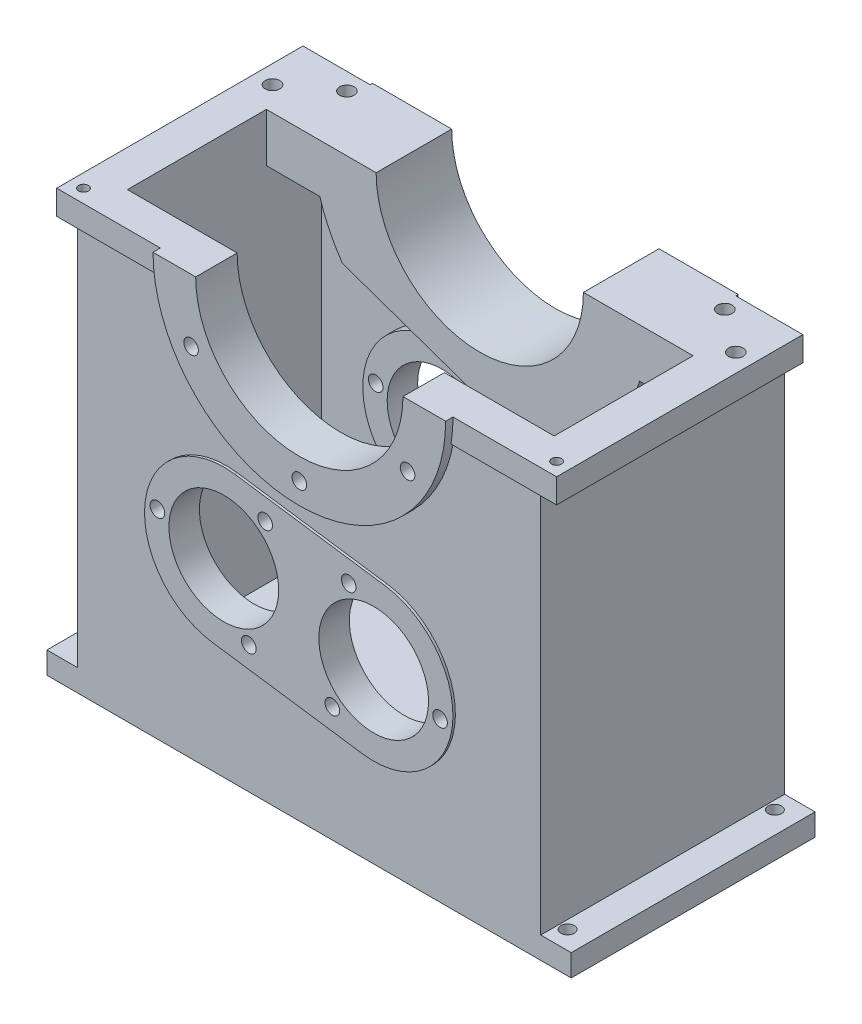
from build123d import *

# Parameters (mm, degrees)
BOSS_EXTRUDE1_DEPTH            = 2
BOSS_EXTRUDE2_DEPTH            = 100
SKETCH3_W                      = 380
SKETCH3_H                      = 200
BOSS_EXTRUDE3_DEPTH            = 232
SKETCH4_W                      = 395
SKETCH4_H                      = 202
BOSS_EXTRUDE4_DEPTH            = 20
SKETCH5_W                      = 202
SKETCH5_H                      = 20
BOSS_EXTRUDE5_DEPTH            = 15
BOSS_EXTRUDE6_START            = 6
BOSS_EXTRUDE6_DEPTH            = 6
SKETCH7_W                      = 200
SKETCH7_H                      = 18
BOSS_EXTRUDE7_DEPTH            = 25
SKETCH8_W                      = 200
SKETCH8_H                      = 18
BOSS_EXTRUDE8_DEPTH            = 25
SKETCH9_W                      = 350
SKETCH9_H                      = 114
CUT_EXTRUDE1_DEPTH             = 337
SKETCH10_W                     = 350
SKETCH10_H                     = 297
CUT_EXTRUDE2_DEPTH             = 45
SKETCH11_W                     = 350
SKETCH11_H                     = 297
CUT_EXTRUDE3_DEPTH             = 11
BOSS_EXTRUDE9_DEPTH            = 2
BOSS_EXTRUDE10_DEPTH           = 45
BOSS_EXTRUDE11_DEPTH           = 11
BOSS_EXTRUDE12_START           = 2
BOSS_EXTRUDE12_DEPTH           = 2
BOSS_EXTRUDE13_START           = 8
BOSS_EXTRUDE13_DEPTH           = 8
BOSS_EXTRUDE14_DEPTH           = 8
F_16_0_16_DIAMETER_HOLE1_D     = 16
F_16_0_16_DIAMETER_HOLE1_DEPTH = 30
F_12_0_12_DIAMETER_HOLE1_D     = 12
F_12_0_12_DIAMETER_HOLE1_DEPTH = 34
HOLE1_D                        = 170
HOLE1_DEPTH                    = 34
HOLE2_D                        = 170
F_11_0_11_DIAMETER_HOLE1_D     = 11
F_11_0_11_DIAMETER_HOLE1_DEPTH = 18
F_12_0_12_DIAMETER_HOLE2_D     = 12
F_12_0_12_DIAMETER_HOLE2_DEPTH = 12
F_8_0_8_DIAMETER_HOLE1_D       = 8
F_8_0_8_DIAMETER_HOLE1_DEPTH   = 12
F_12_0_12_DIAMETER_HOLE3_D     = 12
F_12_0_12_DIAMETER_HOLE3_DEPTH = 15
F_12_0_12_DIAMETER_HOLE4_D     = 12
F_12_0_12_DIAMETER_HOLE4_DEPTH = 25
F_12_0_12_DIAMETER_HOLE5_D     = 12
F_12_0_12_DIAMETER_HOLE5_DEPTH = 31
M80_CLEARANCE_HOLE1_D          = 90
M80_CLEARANCE_HOLE1_DEPTH      = 25
M80_CLEARANCE_HOLE2_D          = 90
FILLET1_R                      = 100


with BuildPart() as part:
    # Sketch1 → Boss-Extrude1 (new body)
    with BuildSketch(Plane.XY.offset(-156.692981355)):
        with BuildLine():
            Line((639.552238246, 214.743963655), (402.909046922, 214.743963655))
            ThreePointArc((402.909046922, 214.743963655), (521.230642584, 114.743963655), (639.552238246, 214.743963655))
        make_face()
    extrude(amount=-BOSS_EXTRUDE1_DEPTH)

    # Sketch2 → Boss-Extrude2 (add)
    with BuildSketch(Plane(origin=(0, 214.743963655, 0), x_dir=(1, 0, 0), z_dir=(0, 1, 0))):
        Polygon((331.230642584, 158.692981355), (521.230642584, 158.692981355), (711.230642584, 158.692981355), (711.230642584, 358.692981355), (331.230642584, 358.692981355), align=None)
    extrude(amount=-BOSS_EXTRUDE2_DEPTH)

    # Sketch3 → Boss-Extrude3 (add)
    with BuildSketch(Plane.XZ.offset(-114.743963655)):
        with Locations((521.230642584, -258.692981355)):
            Rectangle(SKETCH3_W, SKETCH3_H)
    extrude(amount=BOSS_EXTRUDE3_DEPTH)

    # Sketch4 → Boss-Extrude4 (add)
    with BuildSketch(Plane(origin=(0, 214.743963655, 0), x_dir=(-1, 0, 0), z_dir=(0, 1, 0))):
        with Locations((-513.730642584, -257.692981355)):
            Rectangle(SKETCH4_W, SKETCH4_H)
    extrude(amount=BOSS_EXTRUDE4_DEPTH)

    # Sketch5 → Boss-Extrude5 (add)
    with BuildSketch(Plane(origin=(711.230642584, 0, 0), x_dir=(0, 0, -1), z_dir=(1, 0, 0))):
        with Locations((257.692981355, 224.743963655)):
            Rectangle(SKETCH5_W, SKETCH5_H)
    extrude(amount=BOSS_EXTRUDE5_DEPTH)

    # Sketch6 → Boss-Extrude6 (add)
    with BuildSketch(Plane.XY.offset(-156.692981355).offset(BOSS_EXTRUDE6_START)):
        with BuildLine():
            Line((401.230642584, 234.743963655), (641.230642584, 234.743963655))
            ThreePointArc((641.230642584, 234.743963655), (521.230642584, 114.743963655), (401.230642584, 234.743963655))
        make_face()
    extrude(amount=-BOSS_EXTRUDE6_DEPTH)

    # Sketch7 → Boss-Extrude7 (add)
    with BuildSketch(Plane.ZY.offset(-331.230642584)):
        with Locations((-258.692981355, -108.256036345)):
            Rectangle(SKETCH7_W, SKETCH7_H)
    extrude(amount=BOSS_EXTRUDE7_DEPTH)

    # Sketch8 → Boss-Extrude8 (add)
    with BuildSketch(Plane(origin=(711.230642584, 0, 0), x_dir=(0, 0, -1), z_dir=(1, 0, 0))):
        with Locations((258.692981355, -108.256036345)):
            Rectangle(SKETCH8_W, SKETCH8_H)
    extrude(amount=BOSS_EXTRUDE8_DEPTH)

    # Sketch9 → Cut-Extrude1 (cut)
    with BuildSketch(Plane(origin=(0, 234.743963655, 0), x_dir=(-1, 0, 0), z_dir=(0, 1, 0))):
        with Locations((-521.230642584, -241.692981355)):
            Rectangle(SKETCH9_W, SKETCH9_H)
    extrude(amount=-CUT_EXTRUDE1_DEPTH, mode=Mode.SUBTRACT)

    # Sketch10 → Cut-Extrude2 (cut)
    with BuildSketch(Plane.XY.offset(-298.692981355)):
        with Locations((521.230642584, 46.243963655)):
            Rectangle(SKETCH10_W, SKETCH10_H)
    extrude(amount=-CUT_EXTRUDE2_DEPTH, mode=Mode.SUBTRACT)

    # Sketch11 → Cut-Extrude3 (cut)
    with BuildSketch(Plane(origin=(0, 0, -184.692981355), x_dir=(-1, 0, 0), z_dir=(0, 0, -1))):
        with Locations((-521.230642584, 46.243963655)):
            Rectangle(SKETCH11_W, SKETCH11_H)
    extrude(amount=-CUT_EXTRUDE3_DEPTH, mode=Mode.SUBTRACT)

    # Sketch12 → Boss-Extrude9 (add)
    with BuildSketch(Plane(origin=(0, 0, -358.692981355), x_dir=(-1, 0, 0), z_dir=(0, 0, -1))):
        with BuildLine():
            Line((-671.230642584, 234.743963655), (-371.230642584, 234.743963655))
            ThreePointArc((-371.230642584, 234.743963655), (-391.3046853, 159.782335979), (-446.153917567, 104.884480517))
            ThreePointArc((-446.153917567, 104.884480517), (-388.282477918, 41.311262548), (-444.09903009, -24.073522177))
            Line((-444.09903009, -24.073522177), (-567.055445254, -41.605206922))
            ThreePointArc((-567.055445254, -41.605206922), (-632.890089049, -9.110504263), (-626.440608883, 64.023005362))
            ThreePointArc((-626.440608883, 64.023005362), (-615.103761927, 97.778262306), (-629.105405557, 130.51807669))
            ThreePointArc((-629.105405557, 130.51807669), (-660.301154279, 178.53548763), (-671.230642584, 234.743963655))
        make_face()
    extrude(amount=BOSS_EXTRUDE9_DEPTH)

    # Sketch13 → Boss-Extrude10 (add)
    with BuildSketch(Plane.XY.offset(-343.692981355)):
        with BuildLine():
            Line((390.051637579, 194.743963655), (652.409647589, 194.743963655))
            ThreePointArc((652.409647589, 194.743963655), (617.988571356, 137.55428018), (560.64620314, 103.388168426))
            Line((560.64620314, 103.388168426), (408.580498696, 156.527108463))
            ThreePointArc((408.580498696, 156.527108463), (397.827662605, 174.913905269), (390.051637579, 194.743963655))
        make_face()
    extrude(amount=BOSS_EXTRUDE10_DEPTH)

    # Sketch14 → Boss-Extrude11 (add)
    with BuildSketch(Plane(origin=(0, 0, -173.692981355), x_dir=(-1, 0, 0), z_dir=(0, 0, -1))):
        with BuildLine():
            Line((-634.367727574, 194.743963655), (-408.093557595, 194.743963655))
            ThreePointArc((-408.093557595, 194.743963655), (-521.230642584, 114.743963655), (-634.367727574, 194.743963655))
        make_face()
    extrude(amount=BOSS_EXTRUDE11_DEPTH)

    # Sketch15 → Boss-Extrude12 (add)
    with BuildSketch(Plane.XY.offset(-158.692981355).offset(BOSS_EXTRUDE12_START)):
        with BuildLine():
            Line((462.449424751, 104.624818977), (585.405839915, 87.093134232))
            ThreePointArc((585.405839915, 87.093134232), (640.579813161, 13.568766324), (567.055445254, -41.605206922))
            Line((567.055445254, -41.605206922), (444.09903009, -24.073522177))
            ThreePointArc((444.09903009, -24.073522177), (388.925056843, 49.45084573), (462.449424751, 104.624818977))
        make_face()
    extrude(amount=-BOSS_EXTRUDE12_DEPTH)

    # Sketch16 → Boss-Extrude13 (add)
    with BuildSketch(Plane.XY.offset(-343.692981355).offset(BOSS_EXTRUDE13_START)):
        with BuildLine():
            ThreePointArc((517.462463333, 50.516271939), (640.579813161, 13.568766324), (512.042406672, 12.503340115))
            ThreePointArc((512.042406672, 12.503340115), (388.925056843, 49.45084573), (517.462463333, 50.516271939))
        make_face()
    extrude(amount=-BOSS_EXTRUDE13_DEPTH)

    # Sketch17 → Boss-Extrude14 (add)
    with BuildSketch(Plane(origin=(0, 0, -173.692981355), x_dir=(-1, 0, 0), z_dir=(0, 0, -1))):
        with BuildLine():
            ThreePointArc((-512.042406672, 12.503340115), (-640.579813161, 13.568766324), (-517.462463333, 50.516271939))
            ThreePointArc((-517.462463333, 50.516271939), (-388.925056843, 49.45084573), (-512.042406672, 12.503340115))
        make_face()
    extrude(amount=BOSS_EXTRUDE14_DEPTH)

    # Ø16.0 (16) diameter hole1
    with Locations(Plane(origin=(0, 0, -360.692981355), x_dir=(-1, 0, 0), z_dir=(0, 0, -1))):
        with Locations((-421.637721149, 177.243963655), (-620.82356402, 177.243963655)):
            Hole(F_16_0_16_DIAMETER_HOLE1_D / 2, depth=F_16_0_16_DIAMETER_HOLE1_DEPTH)

    # Ø12.0 (12) diameter hole1
    with Locations(Plane(origin=(0, 0, -184.692981355), x_dir=(-1, 0, 0), z_dir=(0, 0, -1))):
        with Locations((-521.230642584, 132.243963655), (-432.463038696, 183.493963655), (-609.998246472, 183.493963655)):
            Hole(F_12_0_12_DIAMETER_HOLE1_D / 2, depth=F_12_0_12_DIAMETER_HOLE1_DEPTH)

    # Hole1
    with Locations(Plane(origin=(0, 0, -184.692981355), x_dir=(-1, 0, 0), z_dir=(0, 0, -1))):
        with Locations((-521.230642584, 234.743963655)):
            Hole(HOLE1_D / 2, depth=HOLE1_DEPTH)

    # Hole2 (through all)
    with Locations(Plane(origin=(0, 0, -360.692981355), x_dir=(-1, 0, 0), z_dir=(0, 0, -1))):
        with Locations((-521.230642584, 234.743963655)):
            Hole(HOLE2_D / 2)

    # Ø11.0 (11) diameter hole1
    with Locations(Plane(origin=(0, -117.256036345, 0), x_dir=(-1, 0, 0), z_dir=(0, -1, 0))):
        with Locations((-718.230642584, 343.692981355), (-324.230642584, 343.692981355), (-324.230642584, 173.692981355), (-718.230642584, 173.692981355)):
            Hole(F_11_0_11_DIAMETER_HOLE1_D / 2, depth=F_11_0_11_DIAMETER_HOLE1_DEPTH)

    # Ø12.0 (12) diameter hole2
    with Locations(Plane(origin=(0, 234.743963655, 0), x_dir=(1, 0, 0), z_dir=(0, 1, 0))):
        with Locations((331.230642584, 318.692981355), (366.230642584, 344.692981355), (711.230642584, 318.692981355), (676.230642584, 344.692981355)):
            Hole(F_12_0_12_DIAMETER_HOLE2_D / 2, depth=F_12_0_12_DIAMETER_HOLE2_DEPTH)

    # Ø8.0 (8) diameter hole1
    with Locations(Plane(origin=(0, 234.743963655, 0), x_dir=(1, 0, 0), z_dir=(0, 1, 0))):
        with Locations((327.230642584, 167.692981355), (715.230642584, 167.692981355)):
            Hole(F_8_0_8_DIAMETER_HOLE1_D / 2, depth=F_8_0_8_DIAMETER_HOLE1_DEPTH)

    # Ø12.0 (12) diameter hole3
    with Locations(Plane.ZY.offset(-331.230642584)):
        with Locations((-257.692981355, -85.256036345)):
            Hole(F_12_0_12_DIAMETER_HOLE3_D / 2, depth=F_12_0_12_DIAMETER_HOLE3_DEPTH)

    # Ø12.0 (12) diameter hole4
    with Locations(Plane.XY.offset(-335.692981355)):
        with Locations((630.679940765, 14.980335144), (542.282493979, -20.528697533), (555.72949301, 73.780253352), (398.82492924, 48.03927691), (487.222376026, 83.548309587), (473.775376995, -10.760641298)):
            Hole(F_12_0_12_DIAMETER_HOLE4_D / 2, depth=F_12_0_12_DIAMETER_HOLE4_DEPTH)

    # Ø12.0 (12) diameter hole5
    with Locations(Plane(origin=(0, 0, -181.692981355), x_dir=(-1, 0, 0), z_dir=(0, 0, -1))):
        with Locations((-630.679940765, 14.980335144), (-555.72949301, 73.780253352), (-542.282493979, -20.528697533), (-398.82492924, 48.03927691), (-473.775376995, -10.760641298), (-487.222376026, 83.548309587)):
            Hole(F_12_0_12_DIAMETER_HOLE5_D / 2, depth=F_12_0_12_DIAMETER_HOLE5_DEPTH)

    # M80 clearance hole1
    with Locations(Plane.XY.offset(-156.692981355)):
        with Locations((453.27422742, 40.2756484), (576.230642584, 22.743963655)):
            Hole(M80_CLEARANCE_HOLE1_D / 2, depth=M80_CLEARANCE_HOLE1_DEPTH)

    # M80 clearance hole2 (through all)
    with Locations(Plane(origin=(0, 0, -360.692981355), x_dir=(-1, 0, 0), z_dir=(0, 0, -1))):
        with Locations((-453.27422742, 40.2756484), (-576.230642584, 22.743963655)):
            Hole(M80_CLEARANCE_HOLE2_D / 2)

    # Fillet1
    fillet1_edges = [part.edges().sort_by_distance(p)[0] for p in [
        (446.153917567, 104.884480517, -359.692981355),
    ]]
    fillet(fillet1_edges, radius=FILLET1_R)


solid = part.part
